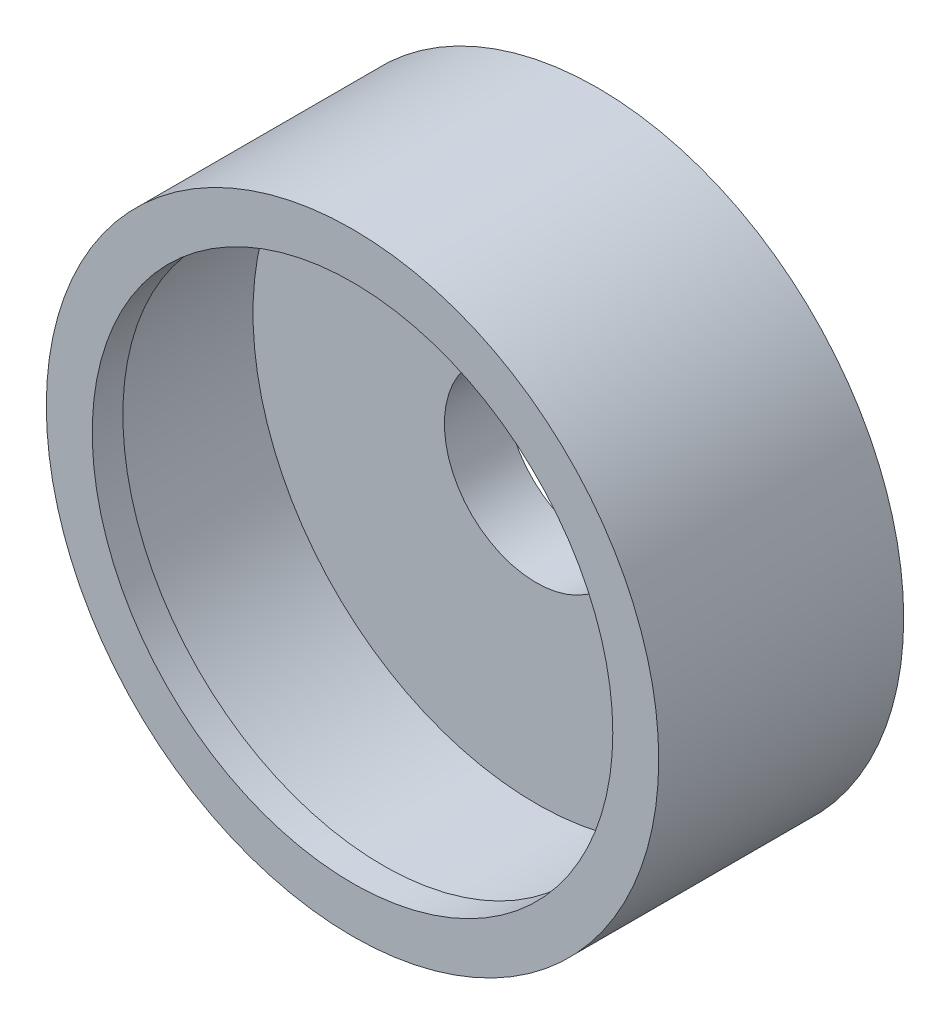
from build123d import *

# Parameters (mm, degrees)
SKETCH1_R           = 10
BOSS_EXTRUDE1_DEPTH = 8
SKETCH2_R           = 8.5
CUT_EXTRUDE1_DEPTH  = 6
SKETCH3_R           = 3
CUT_EXTRUDE2_DEPTH  = 16.362291496
SKETCH4_R           = 9.25
CUT_EXTRUDE3_DEPTH  = 5


with BuildPart() as part:
    # Sketch1 → Boss-Extrude1 (new body)
    with BuildSketch(Plane.XY):
        Circle(SKETCH1_R)
    extrude(amount=BOSS_EXTRUDE1_DEPTH)

    # Sketch2 → Cut-Extrude1 (cut)
    with BuildSketch(Plane.XY.offset(8)):
        Circle(SKETCH2_R)
    extrude(amount=-CUT_EXTRUDE1_DEPTH, mode=Mode.SUBTRACT)

    # Sketch3 → Cut-Extrude2 (cut, through all)
    with BuildSketch(Plane.XY.offset(2)):
        Circle(SKETCH3_R)
    extrude(amount=-CUT_EXTRUDE2_DEPTH, mode=Mode.SUBTRACT)

    # Sketch4 → Cut-Extrude3 (cut)
    with BuildSketch(Plane.XY.offset(2)):
        Circle(SKETCH4_R)
    extrude(amount=CUT_EXTRUDE3_DEPTH, mode=Mode.SUBTRACT)


solid = part.part
